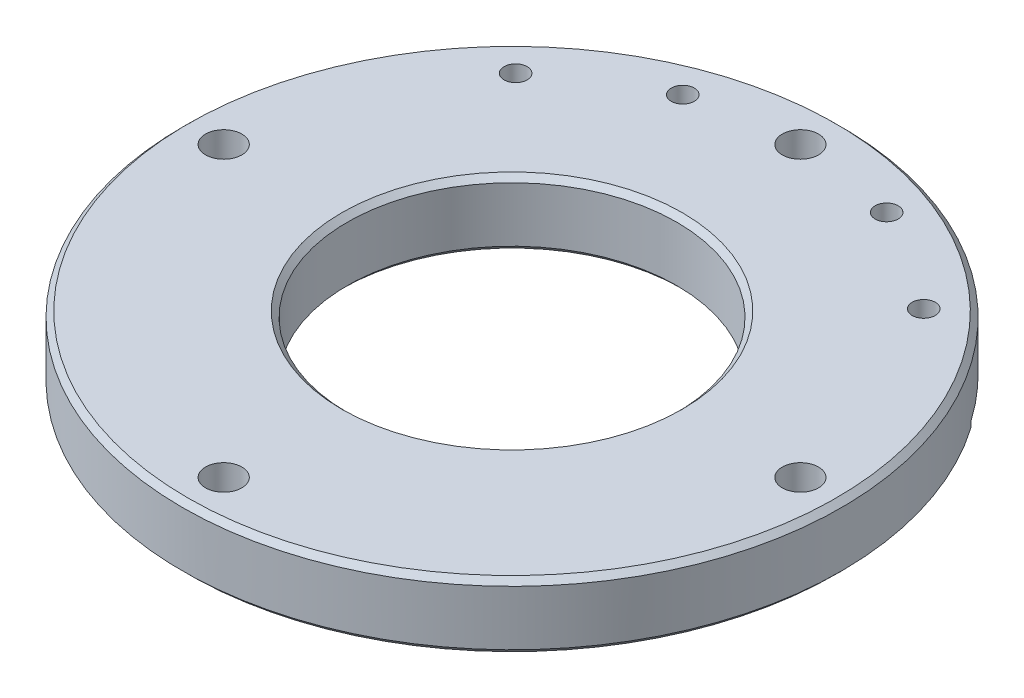
SolidWorks part; units mm, degrees
ref_plane "Front Plane" through (0, 0, 0) normal (0, 0, 1) x (1, 0, 0)
ref_plane "Top Plane" through (0, 0, 0) normal (0, 1, 0) x (1, 0, 0)
ref_plane "Right Plane" through (0, 0, 0) normal (1, 0, 0) x (0, 0, -1)
sketch "Sketch1" plane through (0, 0, 0) normal (0, 1, 0) x (1, 0, 0)
  circle A0 centre (0, 0) radius 60
  circle A1 centre (0, 0) radius 30
  dimension "D1" = 120
  dimension "D2" = 60
extrude "Boss-Extrude1" add sketch "Sketch1" along normal mid plane 12
chamfer "Chamfer1" distance 1 angle 45 4 edges at (0, -6, 30) (0, -6, 60) (0, 6, 30) (0, 6, 60)
hole_wizard "Hole Size by Socket Head Cap Screw Type1" positions "Sketch3" profile "Sketch2" counterbore size "M6" standard "Gb" end condition through all
sketch "Sketch3" plane through (-41.1264, -6, 15.0061) normal (0, 1, 0) x (1, 0, 0)
  line L0 (41.1264, 15.0061) -> (41.1264, 25.4816) construction
  line L2 (41.1264, 15.0061) -> (26.7637, 15.0061) construction
  point P0 (-11.3736, 15.0061)
  point P2 (93.6264, 15.0061)
  point P4 (41.1264, 67.5061)
  point P6 (41.1264, -37.4939)
  dimension "D1" = 105
  dimension "D2" = 105
sketch "Sketch2" plane through (-52.5, -6, 0) normal (1, 0, 0) x (0, 0, -1)
  line L0 (0, 0) -> (0, 12)
  line L1 (0, 12) -> (3.3, 12)
  line L3 (3.3, 12) -> (3.3, 6.8)
  line L4 (3.3, 6.8) -> (5.5, 6.8)
  line L5 (5.5, 6.8) -> (5.5, 0)
  line L7 (5.5, 0) -> (0, 0)
  line L11 (0, -6.35) -> (0, 107.95) construction
  dimension "通孔孔直径" = 6.6
  dimension "通孔孔深度" = 12
  dimension "柱形沉头孔直径" = 11
  dimension "柱形沉头孔深度" = 6.8
sketch "Sketch4" plane through (0, -6, 0) normal (0, -1, 0) x (1, 0, 0)
  line L0 (-37.681, -26.3845) -> (-49.1491, -34.4146)
  line L1 (-7.9878, -45.3012) -> (-10.4189, -59.0885)
  line L2 (7.9878, -45.3012) -> (10.4189, -59.0885)
  line L3 (37.681, -26.3845) -> (49.1491, -34.4146)
  line L4 (0, 0) -> (0, -72.501) construction
  line L5 (0, 0) -> (-7.9878, -45.3012) construction
  line L6 (0, 0) -> (-37.681, -26.3845) construction
  line L7 (0, 0) -> (7.9878, -45.3012) construction
  line L8 (0, 0) -> (37.681, -26.3845) construction
  arc A0 (-37.681, -26.3845) -> (-7.9878, -45.3012) centre (0, 0) ccw
  circle A1 centre (0, 0) radius 60 construction
  arc A2 (-49.1491, -34.4146) -> (-10.4189, -59.0885) centre (0, 0) ccw
  arc A3 (10.4189, -59.0885) -> (49.1491, -34.4146) centre (0, 0) ccw
  arc A4 (7.9878, -45.3012) -> (37.681, -26.3845) centre (0, 0) ccw
  dimension "D1" = 92
  dimension "D2" = 10
  dimension "D3" = 10
  dimension "D4" = 45
  dimension "D5" = 45
extrude "Cut-Extrude1" cut sketch "Sketch4" against normal blind 2
fillet "Fillet1" radius 2 4 edges at (37.681, -5, -26.3845) (7.9878, -5, -45.3012) (-7.9878, -5, -45.3012) (-37.681, -5, -26.3845)
hole_wizard "M5 Tapped Hole1" positions "Sketch6" profile "Sketch5" tap size "M5" standard "Gb" end condition through all
sketch "Sketch6" plane through (0, -4, 0) normal (0, -1, 0) x (-1, 0, 0)
  point P0 (37.1482, 37.8023)
  point P3 (18.561, 49.6436)
  point P6 (-18.561, 49.6436)
  point P9 (-37.1482, 37.8023)
sketch "Sketch5" plane through (-37.1482, -4, -37.8023) normal (1, 0, 0) x (0, 0, -1)
  line L0 (0, 0) -> (0, 10)
  line L1 (0, 10) -> (2.1, 10)
  line L2 (2.1, 10) -> (2.1, 0)
  line L5 (2.1, 0) -> (0, 0)
  line L11 (0, -6.35) -> (0, 107.95) construction
  dimension "通孔螺纹孔钻头直径" = 4.2
  dimension "通孔螺纹孔钻头深度" = 10
cosmetic thread "Hole Cosmetic Thread1" parameters "D2"=5
cosmetic thread "Hole Cosmetic Thread2" parameters "D2"=5
cosmetic thread "Hole Cosmetic Thread3" parameters "D2"=5
cosmetic thread "Hole Cosmetic Thread4" parameters "D2"=5
